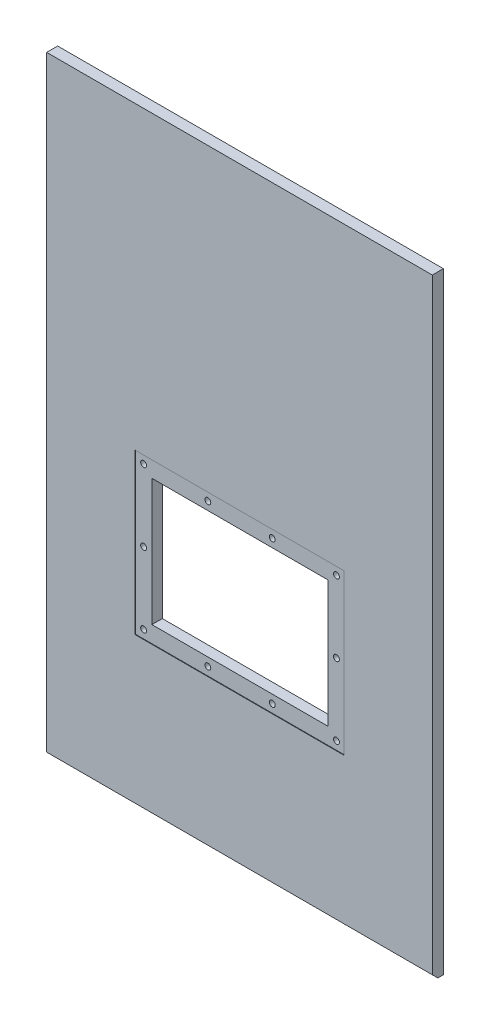
SolidWorks part; units mm, degrees
material "Q235"
ref_plane "Front Plane" through (0, 0, 0) normal (0, 0, 1) x (1, 0, 0)
ref_plane "Top Plane" through (0, 0, 0) normal (0, 1, 0) x (1, 0, 0)
ref_plane "Right Plane" through (0, 0, 0) normal (1, 0, 0) x (0, 0, -1)
sketch "Sketch1" plane through (0, 0, 0) normal (0, 0, 1) x (1, 0, 0)
  line L1 (0, 0) -> (700, 0)
  line L2 (0, 0) -> (0, 1110)
  line L3 (0, 1110) -> (700, 1110)
  line L4 (700, 0) -> (700, 1110)
  line L5 (190, 535) -> (510, 535)
  line L6 (190, 535) -> (190, 305)
  line L7 (190, 305) -> (510, 305)
  line L8 (510, 535) -> (510, 305)
  dimension "D1" = 1110
  dimension "D2" = 700
  dimension "D3" = 320
  dimension "D4" = 230
  dimension "D5" = 535
  dimension "D6" = 190
extrude "Boss-Extrude1" add sketch "Sketch1" along normal blind 20
sketch "Sketch2" plane through (0, 0, 20) normal (0, 0, 1) x (1, 0, 0)
  line L0 (190, 535) -> (190, 305) construction
  line L1 (160, 565) -> (540, 565)
  line L2 (160, 565) -> (160, 275)
  line L3 (160, 275) -> (540, 275)
  line L4 (540, 565) -> (540, 275)
  line L5 (190, 305) -> (510, 305) construction
  dimension "D1" = 380
  dimension "D2" = 290
  dimension "D3" = 30
  dimension "D4" = 30
extrude "Cut-Extrude1" cut sketch "Sketch2" against normal blind 1
hole_wizard "1/2-13 Threaded hole1" positions "3DSketch1" profile "Sketch4" tap size "1/2-13" standard "Progressive"
sketch3d "3DSketch1"
  line L0 (540, 565, 19) -> (160, 565, 19) construction
  line L1 (540, 275, 19) -> (540, 565, 19) construction
  point P0 (175, 550, 19)
  point P2 (291.5, 550, 19)
  point P4 (408.5, 550, 19)
  point P6 (525, 550, 19)
  point P8 (525, 420, 19)
  point P10 (525, 290, 19)
  point P12 (408.5, 290, 19)
  point P14 (291.5, 290, 19)
  point P16 (175, 290, 19)
  point P18 (175, 420, 19)
  dimension "D1" = 350
  dimension "D2" = 260
  dimension "D3" = 130
  dimension "D4" = 117
  dimension "D5" = 116.5
  dimension "D6" = 15
  dimension "D7" = 15
sketch "Sketch4" plane through (175, 550, 19) normal (1, 0, 0) x (0, -1, 0)
  line L0 (0, 0) -> (0, 17.2195)
  line L1 (0, 17.2195) -> (5.3581, 14)
  line L2 (5.3581, 14) -> (5.3581, 0)
  line L5 (5.3581, 0) -> (0, 0)
  line L10 (0, 17.2195) -> (-5.3581, 14) construction
  line L11 (0, -6.35) -> (0, 107.95) construction
  dimension "螺纹孔钻头直径" = 10.7163
  dimension "螺纹孔钻头深度" = 14
  dimension "导头角度" = 118
cosmetic thread "Cosmetic thread11" parameters "D1"=14, "D2"=12.7
cosmetic thread "Cosmetic thread12" parameters "D1"=14, "D2"=12.7
cosmetic thread "Cosmetic thread13" parameters "D1"=14, "D2"=12.7
cosmetic thread "Cosmetic thread14" parameters "D1"=14, "D2"=12.7
cosmetic thread "Cosmetic thread15" parameters "D1"=14, "D2"=12.7
cosmetic thread "Cosmetic thread16" parameters "D1"=14, "D2"=12.7
cosmetic thread "Cosmetic thread17" parameters "D1"=14, "D2"=12.7
cosmetic thread "Cosmetic thread18" parameters "D1"=14, "D2"=12.7
cosmetic thread "Cosmetic thread19" parameters "D1"=14, "D2"=12.7
cosmetic thread "Cosmetic thread20" parameters "D1"=14, "D2"=12.7
chamfer "Chamfer1" distance 10 angle 45 1 edges at (350, 0, 20)
